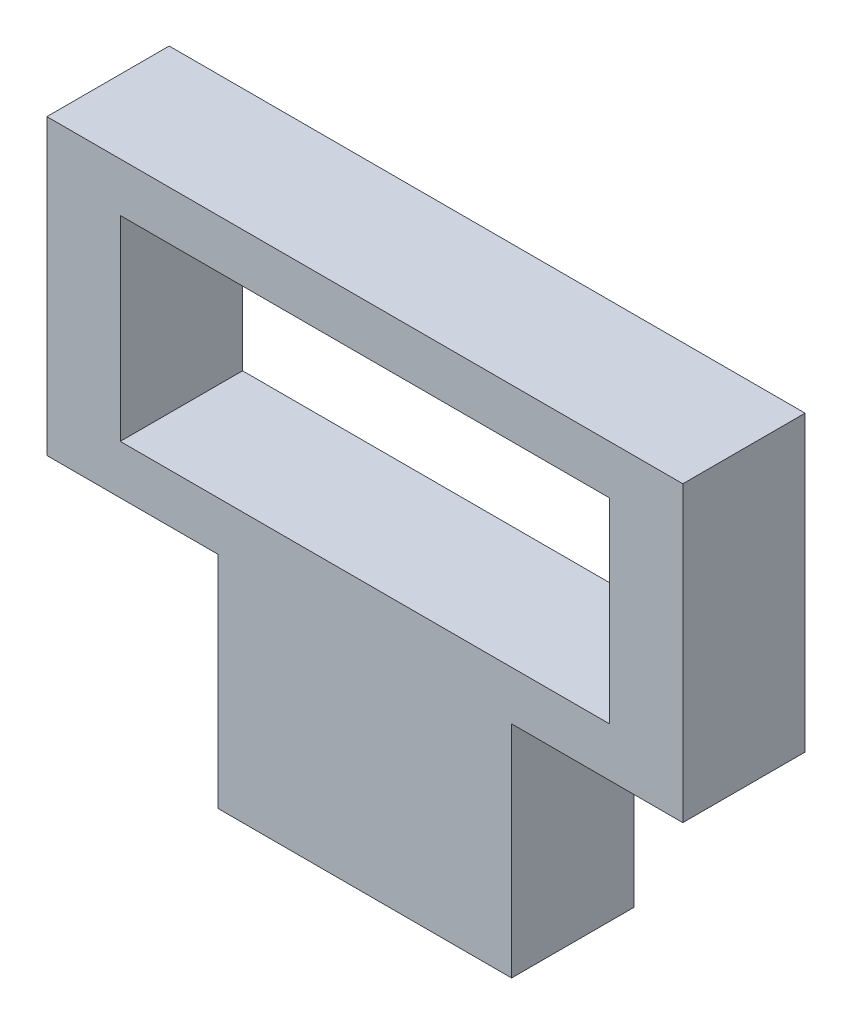
from build123d import *

# Parameters (mm, degrees)
SKETCH_1_W      = 26
SKETCH_1_H      = 12
SKETCH_1_W_2    = 20
SKETCH_1_H_2    = 8
EXTRUDE_1_DEPTH = 2.5
SKETCH_2_W      = 12
SKETCH_2_H      = 9
EXTRUDE_2_DEPTH = 2.5


with BuildPart() as part:
    # 草图1 → 凸台-拉伸1 (new, symmetric)
    with BuildSketch(Plane.XY):
        Rectangle(SKETCH_1_W, SKETCH_1_H)
        Rectangle(SKETCH_1_W_2, SKETCH_1_H_2, mode=Mode.SUBTRACT)
    extrude(amount=EXTRUDE_1_DEPTH, both=True)

    # 草图2 → 凸台-拉伸2 (add, symmetric)
    with BuildSketch(Plane.XY):
        with Locations((0, -10.5)):
            Rectangle(SKETCH_2_W, SKETCH_2_H)
    extrude(amount=EXTRUDE_2_DEPTH, both=True)


solid = part.part
